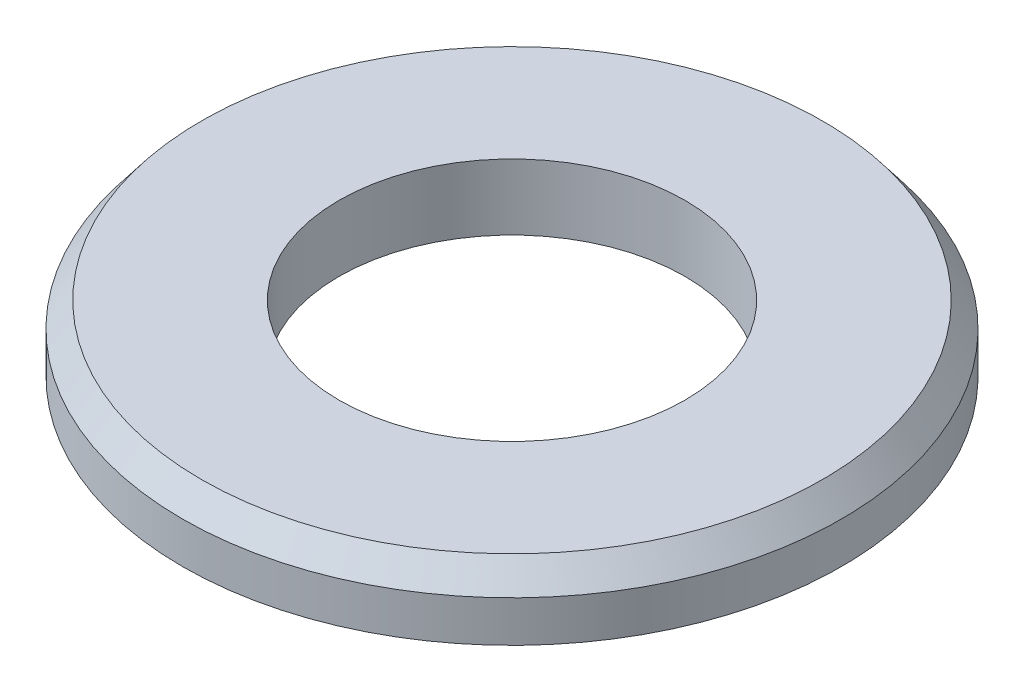
from build123d import *

# Parameters (mm, degrees)
SKETCH1_R           = 10
SKETCH1_R_2         = 5.25
BOSS_EXTRUDE1_DEPTH = 2
CHAMFER1_SIZE       = 0.75
CHAMFER1_SIZE2      = 0.575495241


with BuildPart() as part:
    # Sketch1 → Boss-Extrude1 (new body)
    with BuildSketch(Plane(origin=(0, 0, 0), x_dir=(1, 0, 0), z_dir=(0, 1, 0))):
        with Locations(Location((0, 0, 0), (0, 0, 270))):
            Circle(SKETCH1_R)
        with Locations(Location((0, 0, 0), (0, 0, 270))):
            Circle(SKETCH1_R_2, mode=Mode.SUBTRACT)
    extrude(amount=BOSS_EXTRUDE1_DEPTH)

    # Chamfer1
    chamfer1_edges = [part.edges().sort_by_distance(p)[0] for p in [
        (0, 2, -10),
    ]]
    chamfer1_side = [part.faces().sort_by_distance(p)[0] for p in [
        (0, 1, -10),
    ]]
    chamfer(chamfer1_edges, length=CHAMFER1_SIZE, length2=CHAMFER1_SIZE2, reference=chamfer1_side[0])


solid = part.part
